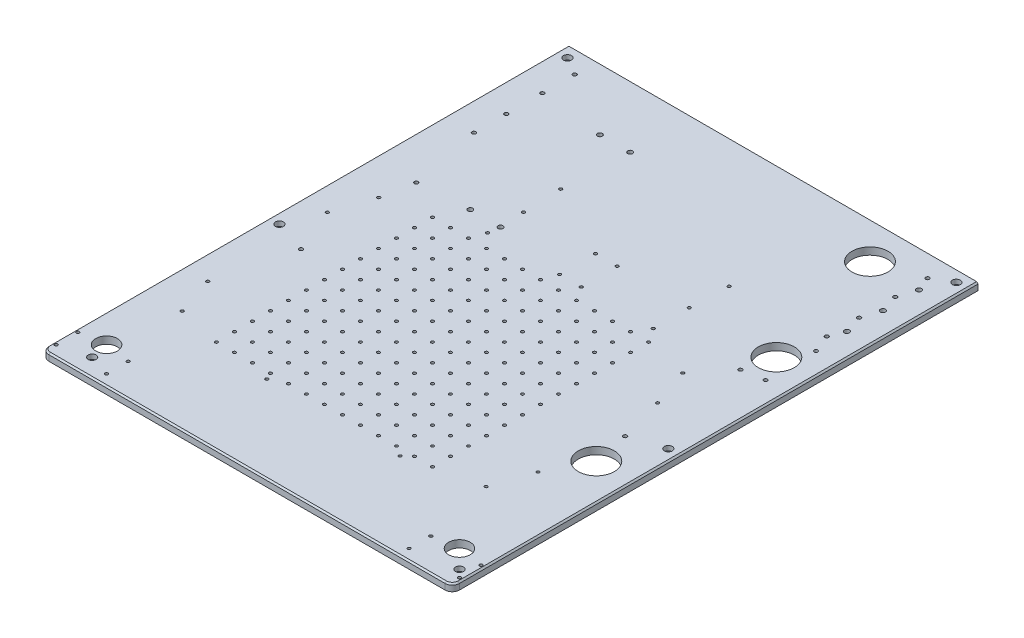
from build123d import *

# Parameters (mm, degrees)
SKETCH_1_W                   = 570
SKETCH_1_H                   = 730
EXTRUDE_1_DEPTH              = 10
FILLET_1_R                   = 10
CHAMFER_1_SIZE               = 2
HOLE_WIZARD_M5_1_D           = 4.2
HOLE_WIZARD_M5_1_DEPTH       = 14
PATTERN_LINEAR_1_COUNT       = 13
PATTERN_LINEAR_1_PITCH       = 25
PATTERN_LINEAR_1_COUNT_DIR2  = 13
PATTERN_LINEAR_1_PITCH_DIR2  = 25
HOLE_WIZARD_M6_1_D           = 6.6
HOLE_WIZARD_M6_1_CBORE_D     = 11
HOLE_WIZARD_M6_1_CBORE_DEPTH = 6.5
HOLE_WIZARD_M8_1_D           = 6.8
HOLE_WIZARD_M8_1_DEPTH       = 22.25
SKETCH_13_R                  = 25
CUT_EXTRUDE_1_DEPTH          = 464.195423121
HOLE_WIZARD_7_0_7_1_D        = 7
HOLE_WIZARD_M6_1_2_D         = 5
HOLE_WIZARD_M5_2_D           = 4.2
SKETCH_21_R                  = 25
CUT_EXTRUDE_2_DEPTH          = 464.195423121
SKETCH_22_R                  = 15
CUT_EXTRUDE_3_DEPTH          = 464.195423121
HOLE_WIZARD_M5_3_D           = 4.2
HOLE_WIZARD_M5_3_DEPTH       = 14
HOLE_WIZARD_M5_3_TIP         = 1.2618073
HOLE_WIZARD_M5_4_D           = 4.2
HOLE_WIZARD_M5_5_D           = 4.2
HOLE_WIZARD_M6_2_D           = 5.2
HOLE_WIZARD_M6_3_D           = 5.2


with BuildPart() as part:
    # 草图1 → 凸台-拉伸1 (new body)
    with BuildSketch(Plane(origin=(0, 0, 0), x_dir=(1, 0, 0), z_dir=(0, 1, 0))):
        Rectangle(SKETCH_1_W, SKETCH_1_H)
    extrude(amount=EXTRUDE_1_DEPTH)

    # 圆角1
    fillet_1_edges = [part.edges().sort_by_distance(p)[0] for p in [
        (285, 5, 365),
        (-285, 5, 365),
    ]]
    fillet(fillet_1_edges, radius=FILLET_1_R)

    # 倒角1
    chamfer_1_edges = [part.edges().sort_by_distance(p)[0] for p in [
        (-285, 10, -5),
        (285, 10, -5),
        (0, 10, 365),
        (-282.071067812, 10, 362.071067812),
        (282.071067812, 10, 362.071067812),
    ]]
    chamfer(chamfer_1_edges, length=CHAMFER_1_SIZE)

    # M5 螺纹孔1
    with Locations(Plane(origin=(0, 10, 0), x_dir=(-1, 0, 0), z_dir=(0, 1, 0))):
        with Locations((172, 235.5)):
            hole_wizard_m5_1 = Hole(HOLE_WIZARD_M5_1_D / 2, depth=HOLE_WIZARD_M5_1_DEPTH)

    # 阵列(线性)1: Hole Wizard M5 _1 13 × 13
    with Locations(*[(i * PATTERN_LINEAR_1_PITCH, 0, -j * PATTERN_LINEAR_1_PITCH_DIR2) for i in range(PATTERN_LINEAR_1_COUNT) for j in range(PATTERN_LINEAR_1_COUNT_DIR2) if (i, j) != (0, 0)]):
        add(hole_wizard_m5_1, mode=Mode.SUBTRACT)

    # Hole Wizard M6 _1 (through all)
    with Locations(Plane(origin=(0, 10, 0), x_dir=(-1, 0, 0), z_dir=(0, 1, 0))):
        with Locations((270, -350), (240, 340), (-270, 340), (-270, -350), (270, 50), (-270, 50)):
            CounterBoreHole(HOLE_WIZARD_M6_1_D / 2, HOLE_WIZARD_M6_1_CBORE_D / 2, HOLE_WIZARD_M6_1_CBORE_DEPTH)

    # M8 螺纹孔1
    with Locations(Plane(origin=(0, 10, 0), x_dir=(-1, 0, 0), z_dir=(0, 1, 0))):
        with Locations((113, -280), (155, -280), (155, -100), (113, -100)):
            Hole(HOLE_WIZARD_M8_1_D / 2, depth=HOLE_WIZARD_M8_1_DEPTH)

    # 草图13 → 切除-拉伸1 (cut, through all)
    with BuildSketch(Plane(origin=(0, 10, 0), x_dir=(1, 0, 0), z_dir=(0, 1, 0))):
        with Locations(Location((185, 315, 0), (0, 0, 270))):
            Circle(SKETCH_13_R)
    extrude(amount=-CUT_EXTRUDE_1_DEPTH, mode=Mode.SUBTRACT)

    # Ø7.0 (7) 直径孔1 (through all)
    with Locations(Plane(origin=(0, 10, 0), x_dir=(-1, 0, 0), z_dir=(0, 1, 0))):
        with Locations((-253, -265), (-253, -315), (-253, -215)):
            Hole(HOLE_WIZARD_7_0_7_1_D / 2)

    # Hole Wizard M6 _1 2 (through all)
    with Locations(Plane(origin=(0, 10, 0), x_dir=(1, 0, 0), z_dir=(0, 1, 0))):
        with Locations((255, 135), (255, 170), (255, 100)):
            Hole(HOLE_WIZARD_M6_1_2_D / 2)

    # M5 螺纹孔2 (through all)
    with Locations(Plane(origin=(0, 10, 0), x_dir=(1, 0, 0), z_dir=(0, 1, 0))):
        with Locations((-251, -2.5), (-251, -168.5), (207.5, -2.5), (207.5, -168.5), (188.95, 51), (188.95, -222), (-233.05, -222), (-233.05, 51), (15, 134), (115, 134), (15, 84), (115, 84), (-15, 134), (-15, 84), (-115, 134), (-115, 84)):
            Hole(HOLE_WIZARD_M5_2_D / 2)

    # 草图21 → 切除-拉伸2 (cut, through all)
    with BuildSketch(Plane(origin=(0, 10, 0), x_dir=(1, 0, 0), z_dir=(0, 1, 0))):
        with Locations(Location((235, 135, 0), (0, 0, 270))):
            Circle(SKETCH_21_R)
        with Locations(Location((235, -115, 0), (0, 0, 270))):
            Circle(SKETCH_21_R)
    extrude(amount=-CUT_EXTRUDE_2_DEPTH, mode=Mode.SUBTRACT)

    # 草图22 → 切除-拉伸3 (cut, through all)
    with BuildSketch(Plane(origin=(0, 10, 0), x_dir=(1, 0, 0), z_dir=(0, 1, 0))):
        with Locations(Location((-245, -315, 0), (0, 0, 270))):
            Circle(SKETCH_22_R)
        with Locations(Location((245, -315, 0), (0, 0, 270))):
            Circle(SKETCH_22_R)
    extrude(amount=-CUT_EXTRUDE_3_DEPTH, mode=Mode.SUBTRACT)

    # M5 螺纹孔3
    with Locations(Plane(origin=(0, 10, 0), x_dir=(1, 0, 0), z_dir=(0, 1, 0))):
        with Locations((210.333452093, -319.740955893), (210, -320), (210, -350), (280, -350), (280, -320)):
            Hole(HOLE_WIZARD_M5_3_D / 2, depth=HOLE_WIZARD_M5_3_DEPTH)
            with Locations((0, 0, -(HOLE_WIZARD_M5_3_DEPTH + HOLE_WIZARD_M5_3_TIP / 2))):  # 118° drill point
                Cone(0, HOLE_WIZARD_M5_3_D / 2, HOLE_WIZARD_M5_3_TIP, mode=Mode.SUBTRACT)

    # M5 螺纹孔4 (through all)
    with Locations(Plane(origin=(0, 10, 0), x_dir=(1, 0, 0), z_dir=(0, 1, 0))):
        with Locations((-280, -320), (-280, -350), (-210, -320), (-210, -350)):
            Hole(HOLE_WIZARD_M5_4_D / 2)

    # M5 螺纹孔5 (through all)
    with Locations(Plane(origin=(0, 10, 0), x_dir=(1, 0, 0), z_dir=(0, 1, 0))):
        with Locations((-92.5, -245), (92.5, -245), (-117, 187.5), (117, 187.5)):
            Hole(HOLE_WIZARD_M5_5_D / 2)

    # M6 螺纹孔2 (through all)
    with Locations(Plane(origin=(0, 10, 0), x_dir=(1, 0, 0), z_dir=(0, 1, 0))):
        with Locations((245, 335), (245, 290), (245, 240), (245, 195), (-245, 335), (-245, 290), (-245, 240), (-245, 195)):
            Hole(HOLE_WIZARD_M6_2_D / 2)

    # M6 螺纹孔3 (through all)
    with Locations(Plane(origin=(0, 10, 0), x_dir=(1, 0, 0), z_dir=(0, 1, 0))):
        with Locations((225, -65), (225, 95), (-225, -65), (-225, 95)):
            Hole(HOLE_WIZARD_M6_3_D / 2)


solid = part.part
